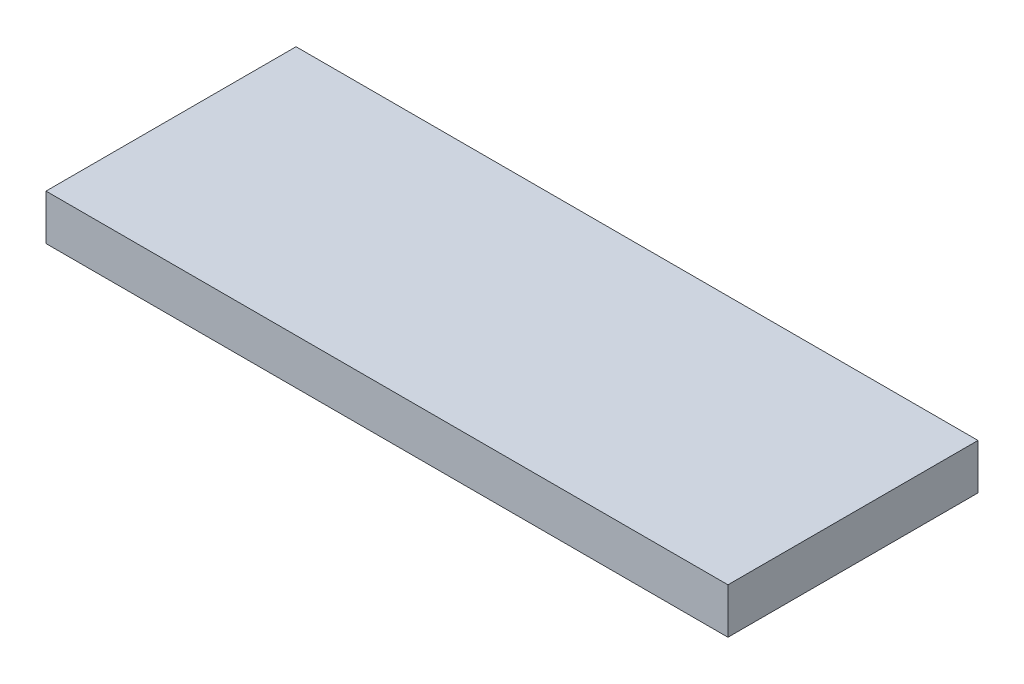
from build123d import *

# Parameters (mm, degrees)
SKETCH_1_W      = 150
SKETCH_1_H      = 10
EXTRUDE_1_DEPTH = 55


with BuildPart() as part:
    # 草图1 → 凸台-拉伸1 (new body)
    with BuildSketch(Plane.XY):
        Rectangle(SKETCH_1_W, SKETCH_1_H)
    extrude(amount=EXTRUDE_1_DEPTH)


solid = part.part
